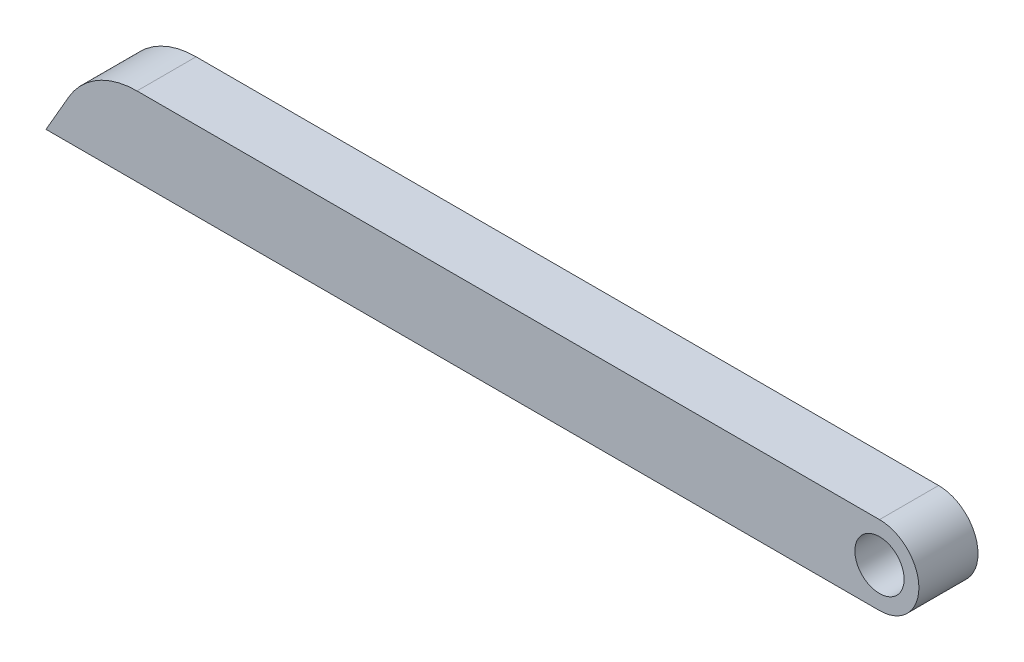
SolidWorks part; units mm, degrees
ref_plane "Front Plane" through (0, 0, 0) normal (0, 0, 1) x (1, 0, 0)
ref_plane "Top Plane" through (0, 0, 0) normal (0, 1, 0) x (1, 0, 0)
ref_plane "Right Plane" through (0, 0, 0) normal (1, 0, 0) x (0, 0, -1)
sketch "Sketch1" plane through (0, 0, 0) normal (0, 0, 1) x (1, 0, 0)
  line L0 (0, 0) -> (20, 0)
  line L1 (20, -2) -> (-1.1547, -2)
  line L2 (-1.1547, -2) -> (0, 0)
  arc A0 (20, 0) -> (20, -2) centre (20, -1) cw
  circle A1 centre (20, -1) radius 0.625
  dimension "D5" = 1
  dimension "D6" = 1.25
  dimension "D1" = 120
  dimension "D3" = 20
extrude "Boss-Extrude2" add sketch "Sketch1" along normal blind 1.5
ref_plane "Plane1" through (0, 0, 0.75) normal (0, 0, -1) x (-1, 0, 0)
sketch "Sketch3" plane through (0, 0, 0.75) normal (0, 0, -1) x (-1, 0, 0)
  line L0 (0.5774, -2) -> (-0.2887, -0.5)
  line L1 (1.1547, -2) -> (-20, -2) construction
  line L2 (-0.2887, -0.5) -> (-1.1547, -0.5)
  line L3 (-1.1547, -0.5) -> (-2.0207, -2)
  line L4 (-2.0207, -2) -> (0.5774, -2)
  line L6 (0, 0) -> (1.1547, -2) construction
  line L7 (-20, 0) -> (0, 0) construction
  circle A0 centre (-0.7217, -1.25) radius 0.75
  circle A1 centre (-0.7217, -1.25) radius 0.4
  dimension "D5" = 0.8
  dimension "D6" = 1.5
  dimension "D1" = 60
  dimension "D2" = 0.5
  dimension "D3" = 0.5
  dimension "D4" = 60
extrude "Cut-Extrude1" cut sketch "Sketch3" against normal mid plane 1 contours A0 L2 L3 | A0 L0 L2 | A0 L4 L0 | A0 L3 L4 | A0 A1
fillet "Fillet1" radius 2 1 edges at (0, 0, 0.75)
